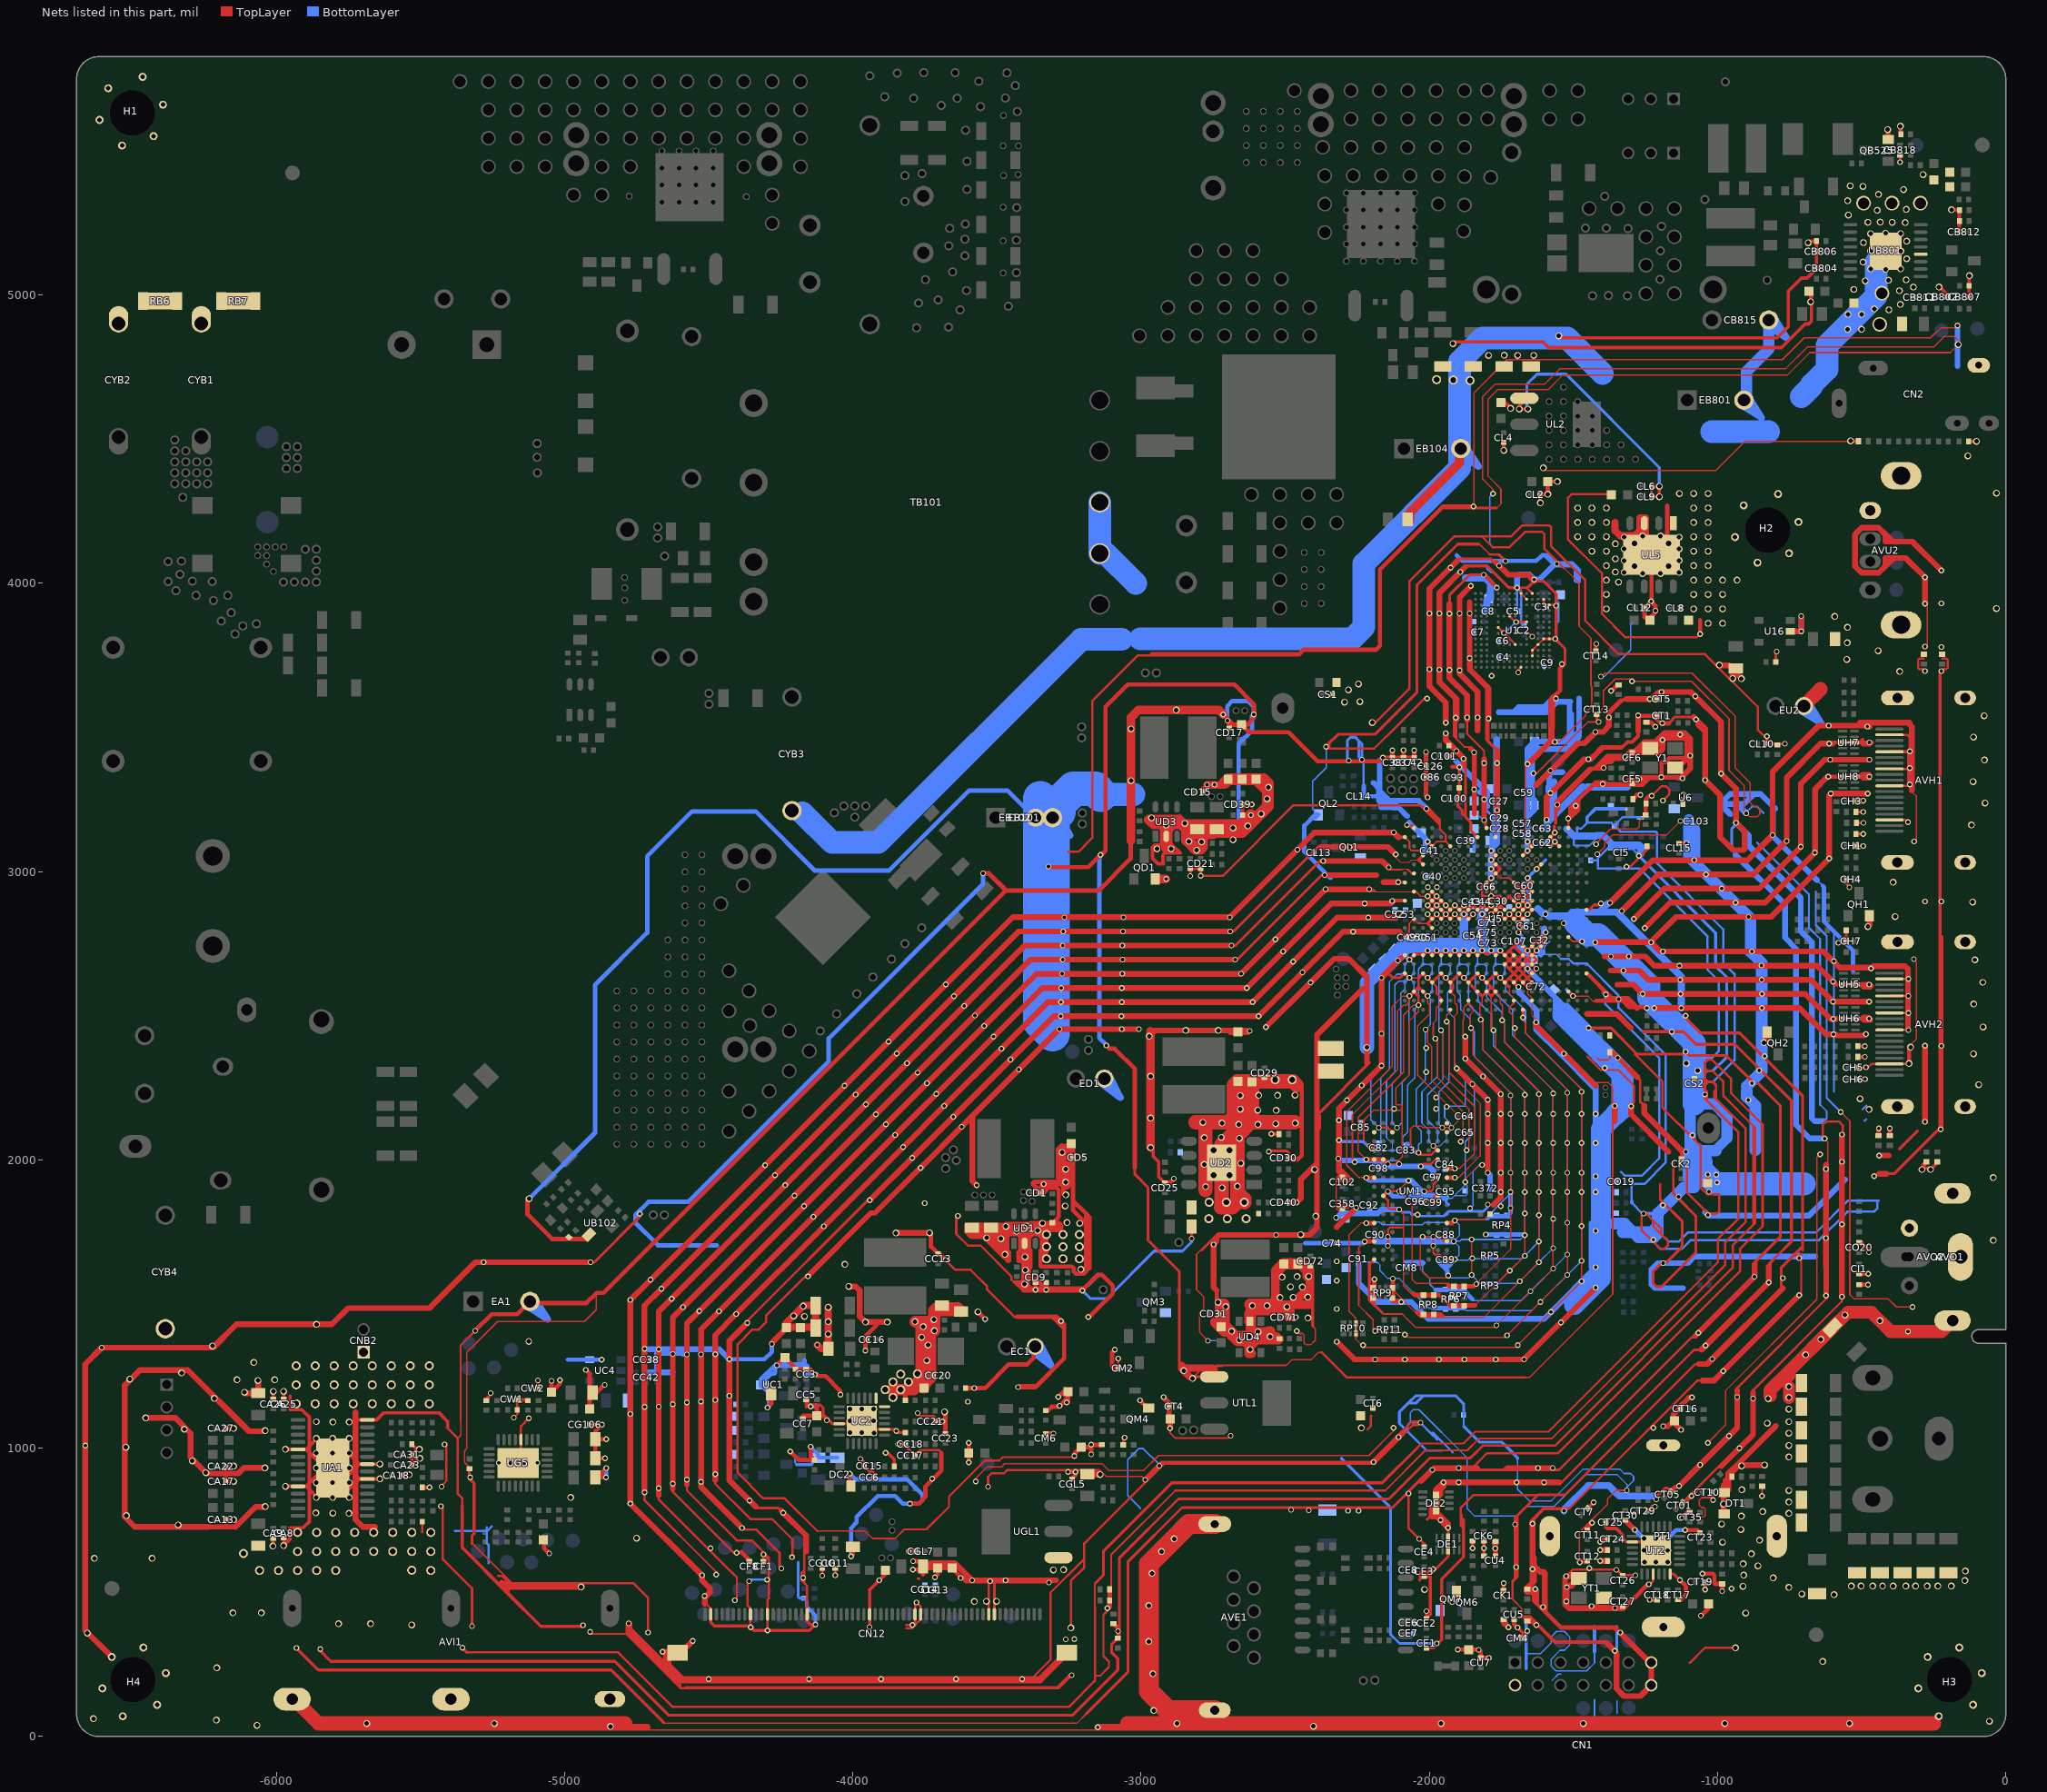
[diagram p0: the nets of this part, all layers, seen from the top]
# Altium PCB MISC84395.PcbDoc (part 14 of 26)
Units mil, origin at the board's own origin, x right, y up, seen from the top; angles counter-clockwise.
Board outline 6692.91 x 5826.77 mil, 2 copper layers (TopLayer, BottomLayer), stack 61.855 mil thick; 951 components, 565 nets, 4374 pads, 1804 vias.
Unrouted connection lines stored in the file: 1.

## Via types
v1: diameter 19.68, hole 11.81, TopLayer to BottomLayer, tented both sides, 1262 vias
v2: diameter 23.62, hole 15.75, TopLayer to BottomLayer, tented both sides, 524 vias
v3: diameter 31.5, hole 19.68, TopLayer to BottomLayer, tented both sides, 11 vias
v4: diameter 24, hole 16, TopLayer to BottomLayer, tented both sides, 6 vias
v5: diameter 19, hole 11.81, TopLayer to BottomLayer, tented both sides, 1 vias

## Nets (pads, with @x,y where several pads share a name; then routed paths per layer and width w, separated by ;. In a path a pad name is that pad's centre, name@x,y a point inside that pad or via, vN(x,y) a via of type N, cw(c..) or ccw(c..) an arc to the next point about the centre after c; other vN are vias at no path point) (continued)
GND: (continued)
  TopLayer w7.8: U1.C4@-1642.97,3747.97 U1.D4@-1642.97,3767.66 U1.E3@-1623.28,3787.34
  TopLayer w7.87: v1(-2175.48,2111.67) -2143.99,2111.67 ; v1(-2143.99,1702.22) -2143.99,1758.32 -2137.1,1765.21 -2096.74,1765.21 ; v1(-2143.99,1891.2) v1(-2104.62,1891.2) ; UM1.B3@-2128.24,2095.93 -2143.99,2111.67 ; UM1.B3@-2128.24,2095.93 -2143.99,2111.67 ; v1(-2104.62,1828.21) -2136.11,1828.21 -2143.99,1836.08 -2143.99,1859.7 ; v1(-2037.69,2025.06) -2029.81,2017.18 -1994.38,2017.18 UM1.D8@-1978.63,2032.93 ; v1(-2037.69,2536.87) -2037.69,2568.36 ; -2037.69,2599.86 -2037.69,2631.36 -2025.24,2643.8 U5.E19@-2021.94,2647.11 ; v1(-2029.81,1977.81) -2021.94,1985.69 -1994.38,1985.69 -1978.63,2001.43 UM1.E8@-1970.75,2001.44 ; v1(-2018,1859.7) -1994.38,1859.7 -1978.63,1875.45 UM1.J8@-1970.75,1875.45 ; v1(-2018,1891.2) -1994.38,1891.2 -1986.51,1899.07 -1986.51,1914.82 -1970.76,1930.57 UM1.G8@-1970.75,1938.45 ; U5.B17@-1958.94,2552.62 -1958.95,2560.49 -1974.69,2576.24 -1974.69,2599.86 ; UM1.T9@-1939.26,1654.98 -1947.14,1654.98 -1962.88,1670.73 -1978.63,1670.73 -1986.51,1678.6 v1(-1986.51,1733.72) -1962.88,1733.72 -1947.14,1717.97 UM1.P9@-1939.26,1717.97 v1(-1915.64,1717.97) ; -2143.99,1859.7 UM1.J2@-2159.73,1875.45 -2143.99,1859.7 ; UM1.D8@-1978.63,2032.93 UM1.D8@-1970.75,2032.93 UM1.D8@-1978.63,2032.93 ; -1974.69,2599.86 U5.D18@-1990.44,2615.61 -1974.69,2599.86
  TopLayer w8: -5493.86,709.08 RA31.1@-5493.86,744.94 ; v1(-5428.91,798.69) -5422.07,791.85 -5422.07,681 ; v1(-5426.23,867) -5426.23,870.14 -5409.97,886.4 v1@-5409.97,1013.74 ; -5422.07,637.12 -5422.07,681 ; -5405.1,1074.37 -5405.1,1068.93 -5370.97,1034.8 -5370.97,842.94 -5355.07,827.03 -5355.07,798.5 ; -5336,292 -4813.44,292 -4813.44,291.29 -4624.65,102.5 -3250.73,102.5 -3159.95,193.27 -3159.95,449.81 ; v1(-5321,383) -5321,514 -5422.07,615.07 -5422.07,681 ; -5230,557.5 -5217.28,557.5 -5191.78,532 ; -5225.79,525.79 -5218.08,533.5 -5193.28,533.5 -5191.78,532 ; v1@-5175,1107 v1(-5176,1106) -5164.27,1117.73 ; RW2.1@-5164.27,1133 -5164.27,1117.73 ; UG5.EPAD@-5161,953.43 -5151.16,963.27 UG5.4@-5151.16,1029.71 -5151.16,1076.84 v1(-5124,1104) ; CW1.1@-5160,1165.73 RG2.1@-5127,1165.73 -5131.27,1170 CW1.1@-5164.27,1170 -5164.27,1117.73 ; CW2.2@-5092.43,1208 v1(-5092.43,1235.43) ; v1(-4777,392) -4780.46,388.54 -4780.46,386.3 -4599.13,204.97 ; v1(-4722.5,847) -4722.5,819.76 -4474,571.26 v1(-4474,562) v1@-4479,562 ; v1(-4710,361) -4710,480.88 -4761.12,532 -5191.78,532 ; -4673.5,838 -4673.5,823.09 -4416.41,566 ; v1@-4656.13,290.13 v1(-4660,294) -4654,288 -4654,261.5 ; -4624.5,859 -4624.5,849.99 -4411.51,637 v1(-4403,637) ; -4615.17,196.97 -4598.36,180.16 -4598.36,168.14 -4580.36,168.14 -4578,170.5 -3292,170.5 -3250.82,211.68 v1@-3241,211.68 ; -4575.5,875 -4575.5,853.32 -4402.31,680.13 -4349.87,680.13 -4291.16,621.42 -4291.16,613.16 ; -4520.49,867.61 -4370.02,717.13 -4334.54,717.13 -4254.16,636.74 -4254.16,589.16 v1(-4248,583) ; -4513.84,460.71 -4508.71,460.71 -4493.03,445.03 CN12.2@-4493.03,423.98 ; -4477.5,890 -4477.5,876.94 -4354.69,754.13 -4280.13,754.13 -4209,683 -4209,624 v1(-4211,622) ; v1@-4402,637 -4388,637 -4382,631 ; -4384.81,643.13 -4382,640.32 ; v1(-4360,539) -4365.84,533.16 -4365.84,455.2 -4355.24,444.59 CN12.9@-4355.24,423.98 -4355.24,380.24 v1(-4354,379) ; CF8.1@-4359,606.57 -4359,612.37 -4359,617.32 ; CF1.1@-4310,606.73 v1(-4310,632) -4291.16,613.16 ; v1@-4297,368 -4296.18,368.82 CN12.12@-4296.18,423.98 -4296.18,473.82 -4291.16,478.84 -4291.16,613.16 ; -4168.16,655.4 -4168.16,577.25 ; v1@-4161.91,1597.91 v1@-4163.95,1595.87 ; CN12.19@-4158.38,423.98 -4158.38,522.38 -4168.16,532.16 ; v1(-4155.69,1595.87) v1@-4163.95,1595.87 ; -4123.13,713.09 -4236.17,826.13 -4310.72,826.13 -4399.5,914.91 -4399.5,1360.32 -4348.48,1411.34 -4326.16,1411.34 -4300.75,1436.75 -4300.75,1459.07 v1@-4163.95,1595.87 ; v1(-4106,558) CG10.1@-4106,584.27 ; v1(-4061,559) CG11.1@-4061,584.27 ; CC18.1@-3817.73,1014 -3817.73,1006.27 -3807.46,996 -3805.28,996 CC17.1@-3784.28,974.99 -3765.43,993.85 -3701.68,993.85 -3696.4,988.57 -3696.4,986.5 -3692.9,983 ; -3815.51,386.49 v1(-3793,386.49) v1@-3793,387 ; -3814,376 -3795,376 -3780,391 ; -3773.76,547.98 -3769.72,547.98 ; v1(-3689,1093) -3679,1083 ; v1(-3678.31,1652.99) -3644.07,1618.75 -3591.53,1618.75 -3535.39,1562.61 -3535.39,1552.03 -3439.36,1456 -3410,1456 ; -3639.63,1741.37 -3601.01,1702.75 -3556.74,1702.75 -3449.84,1595.85 -3449.84,1585.27 ; v1(-3531,867) -3530.81,867.19 -3530.81,900.62 -3518.32,913.11 -3475.79,913.11 -3465.29,923.61 CGL4.1@-3196.5,923.61 ; CN12.51@-3528.46,423.98 -3528.46,534.54 v1(-3524,539) ; -3511,539 -3508.78,536.78 CN12.52@-3508.78,423.98 ; -3441.97,1577.4 -3412.48,1577.4 -3412.4,1577.4 v2(-3404,1569) ; v1(-3412.5,199) v1(-3642,199) v1(-3902,199) v1(-4152,199) v1(-4500,199) -4505.97,204.97 -4599.13,204.97 ; -3253.26,3068.74 -3217.66,3068.74 -3169.84,3116.56 -3169.84,3590.9 -3010.75,3750 -2611,3750 ; v2(-3243.5,377) -3243.5,540.04 -3197,586.54 -3197,669.96 ; -3197,616 -3314.16,498.84 -3314.16,266.38 -3375.57,204.97 -4599.13,204.97 ; CM2.2@-3079.74,1277 v1(-3079.74,1310.74) ; -3027.98,838.98 -3197,669.96 ; v1(-2829.26,2984.26) RD16.1@-2829.26,3010.98 ; CD21.2@-2787.63,3005.35 CD21.2@-2793.26,3010.97 v1(-2793.26,2985.26) -2716.68,2985.26 -2471.62,3230.32 -2032.82,3230.32 -1964.35,3161.85 ; v2@-2558.47,1379.73 -2521.61,1379.73 RD51.1@-2520,1379.73 ; -2374.28,1332.89 -2286.49,1245.11 -1667,1245.11 ; v1(-2358.03,3432.68) -2352.19,3426.84 -2190.49,3426.84 -2107.49,3509.84 -2014.46,3602.88 -2010.88,3602.88 v1(-2008,3600) ; -2214,1066 -2203,1077 -2203,1111 -2201,1113 ; v2(-2198,3517) -2186.6,3517 -2069.88,3633.72 -2069.88,4005.86 -1912.74,4163 -1818.65,4163 ; -2167.88,3783.12 -2167.88,4046.46 -1953.34,4261 -1766,4261 ; -2092.76,1052.76 -2092.76,1060.89 -2060.8,1092.84 -2034.84,1092.84 v1(-2031,1089) -2039,1081 -2056,1081 -2058.26,1078.74 -2191,946 -2920.96,946 -3197,669.96 ; -2073.96,3006.22 -2061.31,2993.56 U5.T20@-2053.43,2993.56 ; v1(-2072.01,842.99) -2072.01,722.36 -2018,668.35 CE4.1@-2018,657.57 ; -2021,3223.84 -2007.58,3223.84 -1964.35,3180.62 -1964.35,3171.35 ; v1(-2010,3218) -2010,3217 -1964.35,3171.35 ; v1(-1990,925) -1549.88,925 -1130.21,1344.67 -1090.17,1384.71 -1084,1384.71 -1078,1390.71 ; -1943.2,3126.55 -1964.35,3147.71 -1964.35,3161.85 ; -1890,731 -1890.81,731.81 -1890.81,794.51 -1848.32,837 -1623.92,837 -1531.64,837 -1077.09,1291.55 -1065.45,1291.55 -1065,1292 ; -1851.64,3700.74 -1795.87,3644.96 -1795.87,3636.48 -1795.87,3459.03 -1796.36,3458.53 -1796.36,3457.12 ; -1851,931.57 -1799.73,982.84 -1553.72,982.84 -1546.47,990.09 -921.5,1615.06 -921.5,1692.69 -844,1770.19 -844,2122.38 -950.32,2228.71 -954.16,2232.54 -954.16,2282.16 -1019,2347 -1035,2347 -1044.8,2337.2 -1044.8,2318.59 ; -1834.29,989.29 -1814.74,1008.84 -1564.49,1008.84 -947.5,1625.83 -947.5,1703.46 -877,1773.96 ; -1829.83,4136 -1828.42,4136 ; -1791.57,4099.16 -1789.45,4099.16 -1758.16,4099.16 -1757.16,4098.16 ; U1.H10@-1759.78,3846.4 U1.H10@-1761.08,3846.4 v1@-1742.52,3827.84 ; v1(-1741.21,3827.84) -1702.02,3788.66 U1.E7@-1702.02,3787.34 ; v1(-1695.65,3984.74) -1695.12,3984.21 -1682.34,3984.21 -1662.67,3984.21 U1.P4@-1642.97,3964.51 ; -1648.5,747.37 -1603.87,792 -1513,792 -1070,1235 -1052.5,1235 ; U1.N2@-1603.6,3944.82 U1.M2@-1603.6,3925.14 U1.M1@-1583.91,3925.14 -1563.3,3925.14 v1(-1560.26,3922.09) ; -1581.36,4099.86 -1600.83,4119.33 ; -1577,876 -1546.55,876 -1081.55,1341 -1056.7,1341 ; v1(-1558,4067) v1@-1558,4076.5 ; -1535.34,4053.84 v1@-1558,4076.5 ; v1(-1525.93,555.93) -1502.7,579.15 v1@-1440.38,579.15 ; U5.AA3@-1518,3151.04 -1518,3183.09 v1@-1518,3183.74 ; v1(-1445.06,583.83) v1@-1440.38,579.15 ; -1399.72,579.12 -1354.18,579.12 v1@-1351.29,576.23 ; -1399.75,579.15 v1@-1440.38,579.15 ; CL5.1@-1371.18,4309 -1505.99,4309 -1519.83,4295.15 -1519.83,4152.88 -1401.15,4034.2 -1401.15,3893.43 -1319.73,3812.02 -1072.82,3812.02 v1(-1060.84,3824) ; v1(-1315.65,3016.74) -1303.51,3016.74 ; -1304.51,3015.74 -1303.51,3016.74 ; -1286.85,2366.9 -1191.99,2272.04 -1191.99,2182.01 -1183.78,2173.8 -1183.78,2173.68 v1@-1087.19,2077.09 ; -1278.46,2286.38 -1267.99,2275.92 -1267.99,2201.41 -1254.99,2188.41 ; v1@-1272.45,3056.06 -1271.58,3055.18 -1271.58,3048.67 -1303.51,3016.74 ; v1(-1228.77,3262.74) -1196.27,3295.24 -1178.6,3295.24 -1167.16,3283.8 -1167.16,3268.2 v1(-1189.56,3245.79) v1@-1190.97,3245.79 ; v1@-1221.84,1724.2 -1223,1725.35 v1(-1223,1723) v1@-1223,1715.35 ; -1198.84,1916 -1198.84,1861.95 -1197.84,1860.95 ; -1153.84,1990 -1153.84,1883.42 -1150.84,1880.42 ; CT01.1@-1121.17,812.83 -1120.45,812.83 -999.12,934.15 ; -1106.16,1971 -1106.16,1946.33 -1106.15,1886.64 v1@-1032.67,1813.16 ; -1096.46,255.46 -1043.92,308 v2(-938,308) ; v1(-1087.19,2085.35) v1@-1087.19,2077.09 ; v1@-1041.16,1813.16 v1@-1032.67,1813.16 ; -1039.03,2276.97 -1032.85,2270.79 -1016.33,2270.79 ; -1032.85,2308.47 -1034.69,2308.47 ; v1(-1030,1889) -1021.84,1880.84 ; -1022.13,2190.2 -1044.8,2212.88 v1@-1044.8,2227.8 ; -999.5,1647.37 -999.5,1725 -929,1795.5 -929,2097.08 -1037.74,2205.82 v1@-1037.74,2220.74 ; -973.89,950.89 -986.73,938.06 ; -973.5,1636.6 -973.5,1714.23 -903,1784.73 -903,2107.85 -1006.16,2211 ; v1(-932.25,1177) -932.25,1209.2 -621,1520.45 -621,1538.99 ; v1(-877.25,1172) -877.25,1201.39 -569,1509.64 v1(-569,1525) ; CL10.1@-829.11,3443 v1(-766.83,3443) ; CL10.1@-829.11,3445 -829.11,3460.27 -861.15,3492.31 -861.15,3571.63 -1043.54,3754.02 -1343.76,3754.02 -1459.15,3869.41 -1459.15,4010.17 -1577.83,4128.86 -1577.83,4194.83 -1584,4201 -1677.81,4201 -1715.81,4163 -1818.65,4163 ; -774,1554.41 -778.5,1558.91 -778.5,1626.99 -778.5,1627.7 -738.11,1668.09 -737.4,1668.09 -716.84,1668.09 -712,1663.25 v1@-711,1662.25 ; v1(-629,2074.13) -635,2080.13 -635,2124.5 -626.5,2133 -579.22,2133 -566,2119.78 v1@-566,2090.87 ; v1@-568.84,2088.02 v1@-566,2090.87 ; v1@-566,2090.81 v1@-566,2090.87 ; CH3.1@-519.92,3244.29 -513.91,3244.29 -497.11,3244.29 v1(-495.21,3246.19) ; v1@-486.37,2319.87 -479.37,2319.87 -466.57,2332.68 AVH2.17@-403.84,2332.68 -337.32,2332.68 v2(-336,2334) ; AVH2.11@-403.84,2450.79 -339.63,2450.79 v1@-338.45,2450.79 ; AVH2.8@-403.84,2509.84 -339.63,2509.84 v1@-338.45,2509.84 ; AVH2.5@-403.84,2568.9 -339.63,2568.9 v1@-338.45,2568.9 ; AVH2.2@-403.84,2627.95 -339.63,2627.95 -338.45,2627.95 v1(-338.37,2627.87) ; AVH1.17@-403.84,3179.13 -348.35,3179.13 -340.37,3171.16 v1(-339.37,3171.16) ; AVH1.11@-403.84,3297.24 v1@-337.92,3297.24 ; AVH1.8@-403.84,3356.3 v1@-334.67,3356.3 ; AVH1.2@-403.84,3474.41 -342.62,3474.41 -333.38,3465.16 ; -375.98,3512.28 -344.37,3512.28 ; v1@-287,3702.41 -300.41,3702.41 -304.22,3706.22 -304.22,3733.9 -299.99,3738.13 -286,3738.13 ; v1(-223.83,3695.57) -216.99,3702.41 -206.61,3702.41 -201.34,3707.68 -201.34,3732.85 -206.61,3738.13 -220,3738.13 ; -4382,631 -4368.32,617.32 -4363.95,617.32 -4359,617.32 ; -4382,631 -4382,635.37 -4382,640.32 ; -4382,640.32 -4359,617.32 ; -4168.16,532.16 -4178.26,542.26 -4178.26,567.16 -4168.16,577.25 ; -4168.16,532.16 -4168.16,577.25 ; v1@-3793,387 -3784.37,395.63 CN12.38@-3784.37,423.98 -3784.37,459.63 v1(-3779,465) -3764.68,450.68 CN12.39@-3764.68,423.98 -3764.68,406.25 -3783.93,387 v1@-3793,387 ; -1964.35,3161.85 -1964.35,3171.35 ; -1818.65,4163 -1780.8,4125.16 -1721.13,4125.16 -1668.29,4178 -1609,4178 -1600.83,4169.83 -1600.83,4119.33 ; -1600.83,4119.33 v1@-1558,4076.5 ; v1@-1223,1715.35 -1199.8,1692.16 -1184.2,1692.16 -1172.92,1703.43 -1172.92,1718.87 -1195.84,1741.79 ; v1@-1223,1715.35 -1264.67,1757.03 -1264.67,1806.33 v1(-1257,1814) -1248.03,1814 -1223,1788.97 ; -1223,1788.97 -1223,1768.95 -1195.84,1741.79 ; -1223,1788.97 -1195.84,1761.81 -1195.84,1741.79 ; v1@-1087.19,2077.09 -1059.16,2049.06 -1059.16,1903.28 -1036.72,1880.84 -1021.84,1880.84 ; v1@-1044.8,2227.8 v1(-1044,2227) v1@-1037.74,2220.74 ; v1@-1044.8,2227.8 -1044.8,2271 ; -1044.8,2271 -1043.65,2269.84 -1033.65,2269.84 ; -1044.8,2271 -1044.8,2281 ; -1044.8,2281 -1044.8,2298.36 ; -1044.8,2281 -1033.65,2269.84 ; -1044.8,2298.36 -1044.8,2318.59 ; -1044.8,2298.36 -1034.69,2308.47 ; -1044.8,2318.59 -1034.69,2308.47 ; v1@-1037.74,2220.74 -1037.74,2237.09 -1043.84,2243.2 -1043.84,2258.8 -1032.8,2269.84 ; -1034.69,2308.47 -1017.24,2308.47 -980.16,2271.39 -980.16,2221.77 -877,2118.62 ; -1033.65,2269.84 -1032.8,2269.84 ; -1032.8,2269.84 -1017.2,2269.84 -1016.33,2268.97 ; v1@-1032.67,1813.16 -1003.26,1813.16 -994.42,1822 -994.42,1878 -997.26,1880.84 -1021.84,1880.84 ; -1016.33,2268.97 -1016.33,2270.79 ; -1016.33,2268.97 -1006.16,2258.8 ; -1016.33,2270.79 -1006.16,2260.62 -1006.16,2258.8 ; -1006.16,2211 -1011.68,2216.52 -1011.68,2237.68 -1006.16,2243.2 ; -1006.16,2211 -1006.16,2243.2 ; -1006.16,2243.2 -1006.16,2258.8 ; -999.12,934.15 -990.64,934.15 -986.73,938.06 ; -999.12,934.15 -995.22,938.06 -986.73,938.06 ; -877,1773.96 -870,1780.96 -870,1810 ; -877,1773.96 -877,1788.82 -877,1812 ; -877,1812 -872,1812 -870,1810 ; -877,1812 -877,2118.62 ; -877,2118.62 -870,2111.61 -870,1810
  TopLayer w9: v1@-1701.54,3866.08 U1.J5@-1662.65,3866.08
  TopLayer w9.8: v1@-1692.21,3697.46 -1682.34,3707.33 U1.A6@-1682.34,3708.6 ; U1.F2@-1603.6,3807.03 U1.F1@-1583.91,3807.03 v1@-1563.89,3807.03
  TopLayer w9.84: UM1.T1@-2191.23,1654.98 -2207.96,1638.26 -2207.96,1513.84 -2162.65,1468.53